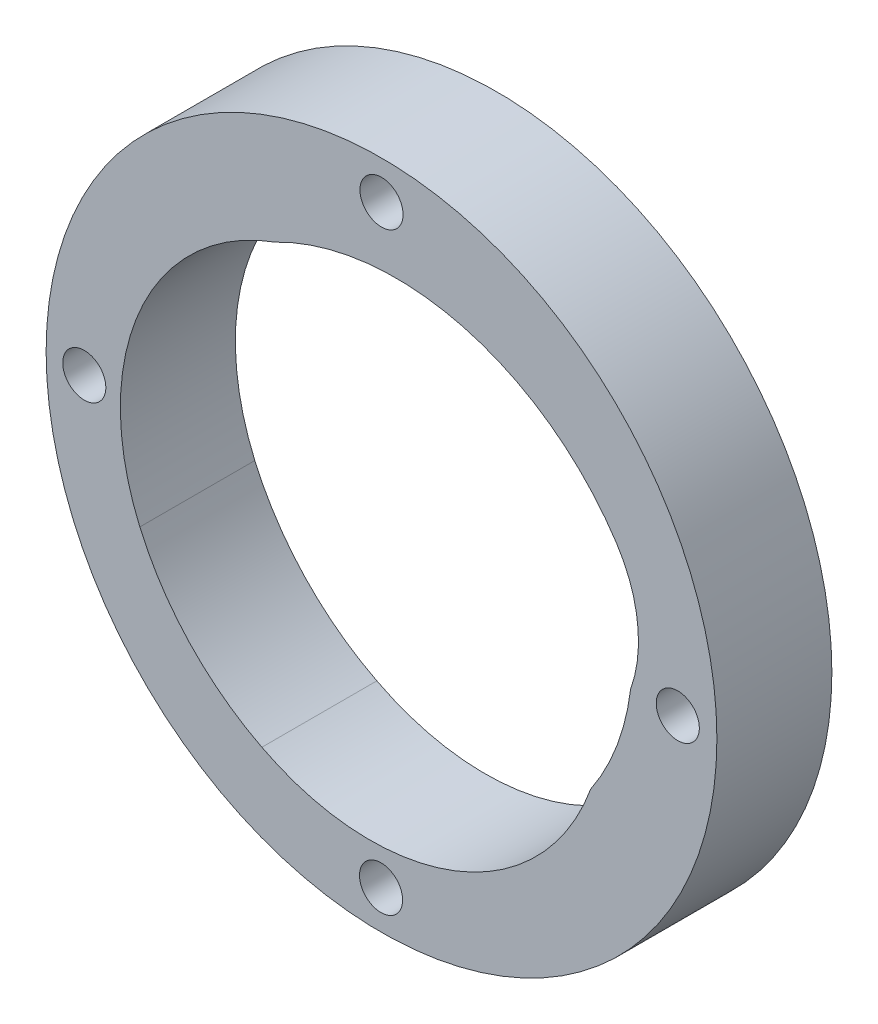
from build123d import *

# Parameters (mm, degrees)
SKETCH_2_R          = 35
EXTRUDE_1_DEPTH     = 12
SKETCH_3_R          = 2.25
CUT_EXTRUDE_1_DEPTH = 51.931326313


with BuildPart() as part:
    # 草图2 → 凸台-拉伸1 (new body)
    with BuildSketch(Plane.XY):
        Circle(SKETCH_2_R)
        with BuildLine():
            ThreePointArc((-12.484738743, -24.502679415), (-20.031862375, -18.840766699), (-25.22108467, -10.961153593))
            ThreePointArc((-25.22108467, -10.961153593), (-25.259217651, 8.481414129), (-11.122767244, 21.829659843))
            ThreePointArc((-11.122767244, 21.829659843), (8.485416214, 24.001994273), (24.502679415, 12.484738743))
            ThreePointArc((24.502679415, 12.484738743), (26.716793299, 6.418124257), (26, 0))
            ThreePointArc((26, 0), (24.576877243, -5.809609847), (21.829659843, -11.122767244))
            ThreePointArc((21.829659843, -11.122767244), (9.253297944, -24.916386782), (-9.389722524, -25.847303746))
            ThreePointArc((-9.389722524, -25.847303746), (-10.960408212, -25.228341041), (-12.484738743, -24.502679415))
        make_face(mode=Mode.SUBTRACT)
    extrude(amount=EXTRUDE_1_DEPTH)

    # 草图3 → 切除-拉伸1 (cut, through all)
    with BuildSketch(Plane.XY.offset(12)):
        with Locations((0, 31)):
            Circle(SKETCH_3_R)
        with Locations((30.917947145, 0.049389692)):
            Circle(SKETCH_3_R)
        with Locations((-0.047414981, -30.978569044)):
            Circle(SKETCH_3_R)
        with Locations((-31.016726529, -0.148169076)):
            Circle(SKETCH_3_R)
    extrude(amount=-CUT_EXTRUDE_1_DEPTH, mode=Mode.SUBTRACT)


solid = part.part
